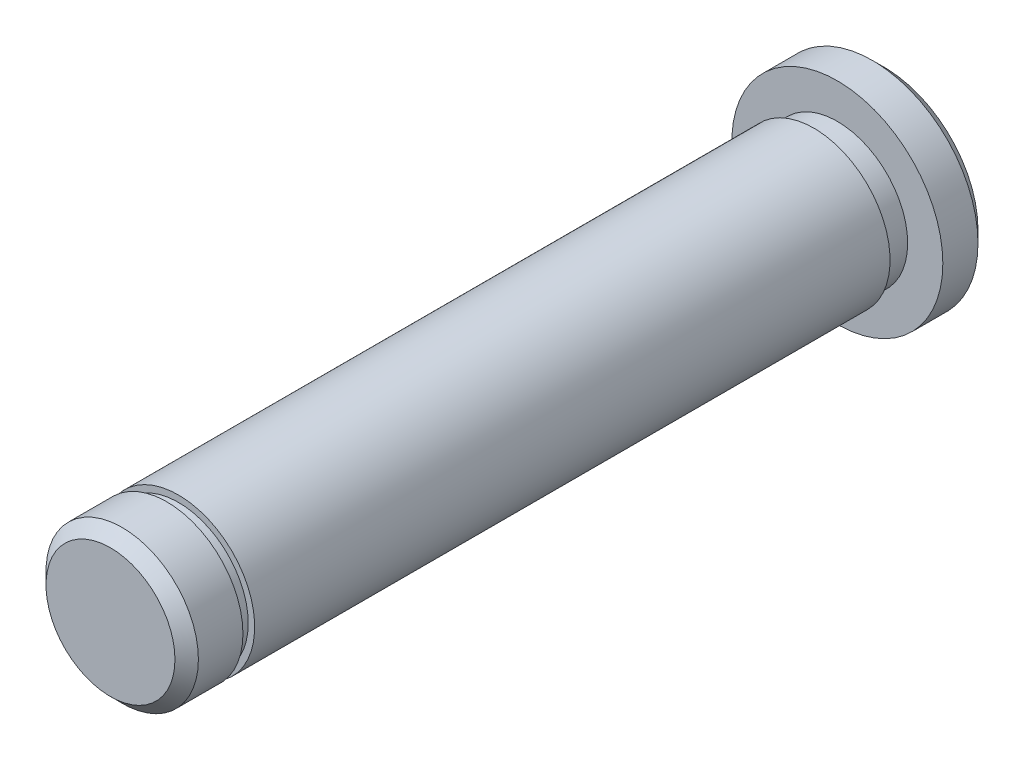
SolidWorks part; units mm, degrees
ref_plane "Front Plane" through (0, 0, 0) normal (0, 0, 1) x (1, 0, 0)
ref_plane "Top Plane" through (0, 0, 0) normal (0, 1, 0) x (1, 0, 0)
ref_plane "Right Plane" through (0, 0, 0) normal (1, 0, 0) x (0, 0, -1)
other "Configuration Table"
sketch "Sketch1" plane through (0, 0, 0) normal (0, 0, 1) x (1, 0, 0)
  circle A0 centre (0, 0) radius 9
  dimension "D1" = 18
extrude "Boss-Extrude1" add sketch "Sketch1" along normal blind 4
sketch "Sketch2" plane through (0, 0, 4) normal (0, 0, 1) x (1, 0, 0)
  circle A0 centre (0, 0) radius 6
  dimension "D1" = 12
extrude "Boss-Extrude2" add sketch "Sketch2" along normal blind 2
sketch "Sketch3" plane through (0, 0, 6) normal (0, 0, 1) x (1, 0, 0)
  circle A0 centre (0, 0) radius 6.5
  dimension "D1" = 13
extrude "Boss-Extrude3" add sketch "Sketch3" along normal blind 54.2
sketch "Sketch4" plane through (0, 0, 60.2) normal (0, 0, 1) x (1, 0, 0)
  circle A0 centre (0, 0) radius 5.95
  dimension "D1" = 11.9
extrude "Boss-Extrude4" add sketch "Sketch4" along normal blind 1
sketch "Sketch5" plane through (0, 0, 61.2) normal (0, 0, 1) x (1, 0, 0)
  circle A0 centre (0, 0) radius 6.5
  dimension "D1" = 13
extrude "Boss-Extrude5" add sketch "Sketch5" along normal offset from surface (4.8 mm away) 66 up to face at (9, 0, 0)
chamfer "Chamfer1" distance 1 angle 45 2 edges at (9, 0, 0) (6.5, 0, 66)
